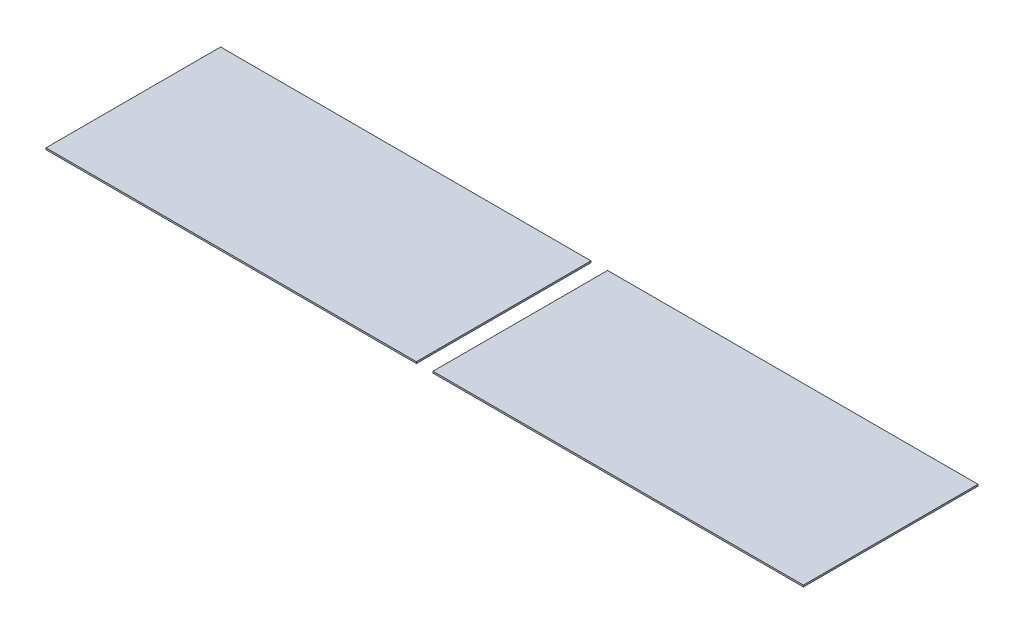
from build123d import *

# Parameters (mm, degrees)
SKETCH1_W           = 1822
SKETCH1_H           = 420
BOSS_EXTRUDE1_DEPTH = 4
SKETCH7_W           = 40
SKETCH7_H           = 573.776848342
CUT_EXTRUDE5_DEPTH  = 935.899459835


with BuildPart() as part:
    # Sketch1 → Boss-Extrude1 (new body)
    with BuildSketch(Plane(origin=(0, 0, 0), x_dir=(1, 0, 0), z_dir=(0, 1, 0))):
        Rectangle(SKETCH1_W, SKETCH1_H)
    extrude(amount=BOSS_EXTRUDE1_DEPTH)

    # Sketch7 → Cut-Extrude5 (cut, through all)
    with BuildSketch(Plane(origin=(0, 4, 0), x_dir=(1, 0, 0), z_dir=(0, 1, 0))):
        Rectangle(SKETCH7_W, SKETCH7_H)
    extrude(amount=-CUT_EXTRUDE5_DEPTH, mode=Mode.SUBTRACT)


with BuildPart() as cut_extrude5_piece_1:
    # of the separate pieces the step leaves, piece 1, a body of its own (cut_extrude5_pieces)
    add(part.part.solids().sort_by_distance((-911, 0, -210))[0])


with BuildPart() as cut_extrude5_piece_2:
    # of the separate pieces the step leaves, piece 2, a body of its own (cut_extrude5_pieces)
    add(part.part.solids().sort_by_distance((20, 0, -210))[0])


solid = Compound([cut_extrude5_piece_1.part, cut_extrude5_piece_2.part])
